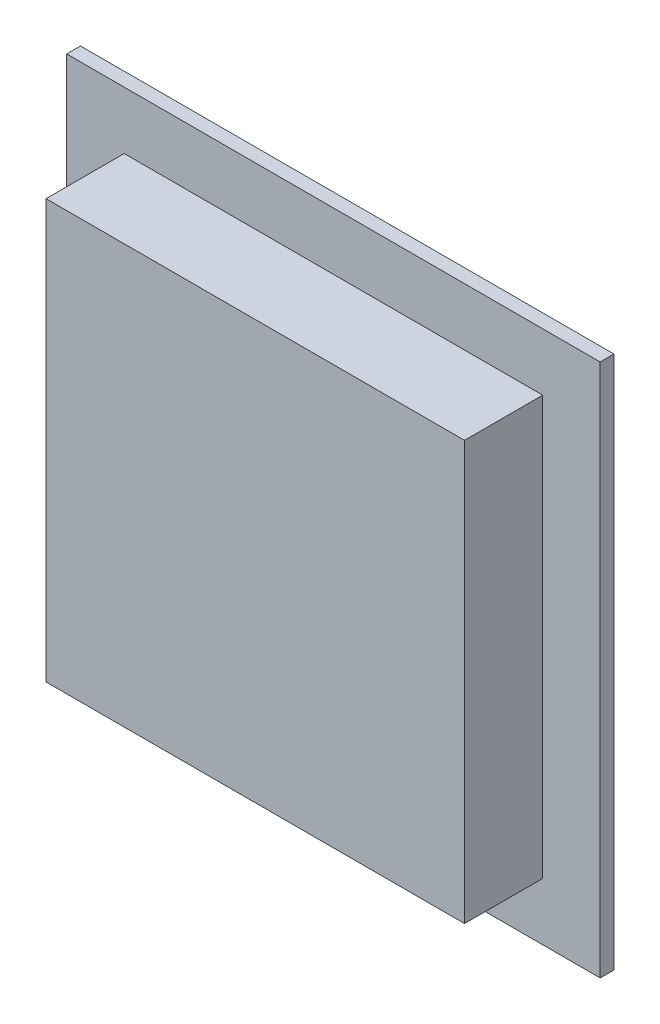
from build123d import *

# Parameters (mm, degrees)
SKETCH_1_W      = 116
SKETCH_1_H      = 116
EXTRUDE_1_DEPTH = 3
SKETCH_2_W      = 91
SKETCH_2_H      = 91
EXTRUDE_2_DEPTH = 17


with BuildPart() as part:
    # 草图1 → 凸台-拉伸1 (new body)
    with BuildSketch(Plane.XY):
        Rectangle(SKETCH_1_W, SKETCH_1_H)
    extrude(amount=EXTRUDE_1_DEPTH)

    # 草图2 → 凸台-拉伸2 (add)
    with BuildSketch(Plane.XY.offset(3)):
        Rectangle(SKETCH_2_W, SKETCH_2_H)
    extrude(amount=EXTRUDE_2_DEPTH)


solid = part.part
